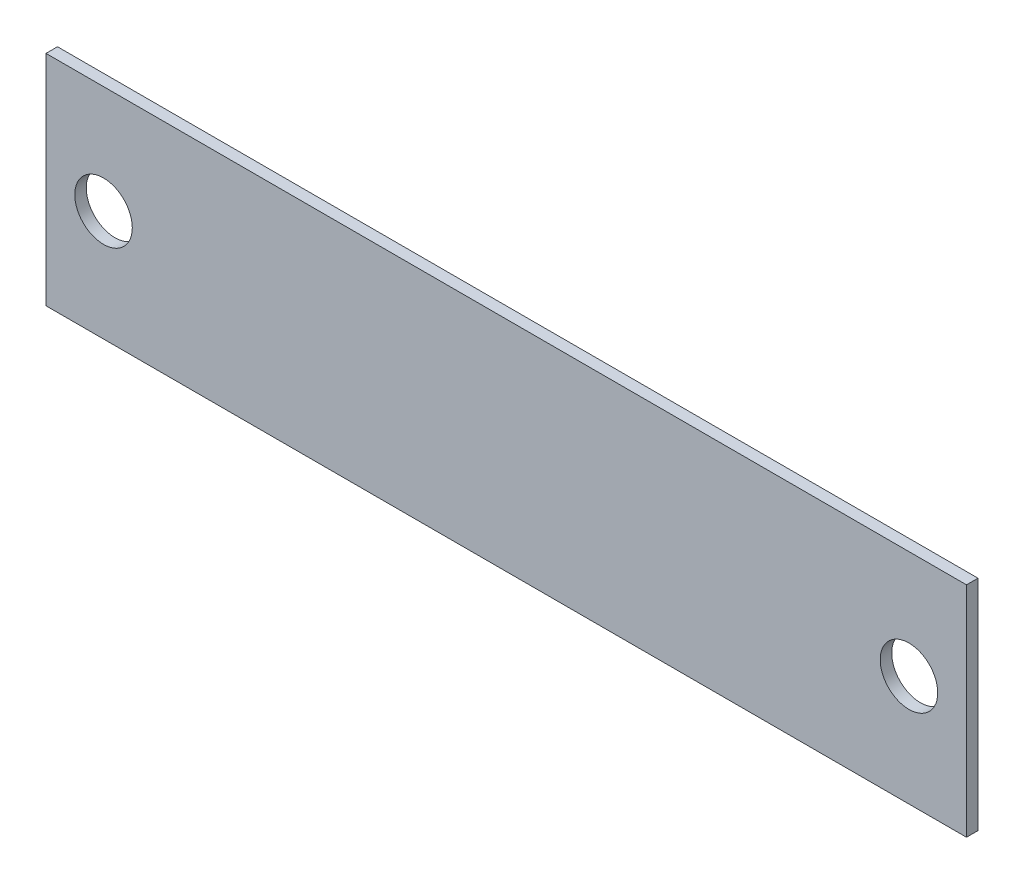
from build123d import *

# Parameters (mm, degrees)
SKETCH_1_W            = 80
SKETCH_1_H            = 19
EXTRUDE_1_DEPTH       = 1
HOLE_WIZARD_5_0_5_1_D = 5


with BuildPart() as part:
    # 草图1 → 凸台-拉伸1 (new body)
    with BuildSketch(Plane.XY):
        with Locations((0, 9.5)):
            Rectangle(SKETCH_1_W, SKETCH_1_H)
    extrude(amount=EXTRUDE_1_DEPTH)

    # Ø5.0 (5) 直径孔1 (through all)
    with Locations(Plane.XY.offset(1)):
        with Locations((-35, 9.621851999), (35, 9.621851999)):
            Hole(HOLE_WIZARD_5_0_5_1_D / 2)


solid = part.part
